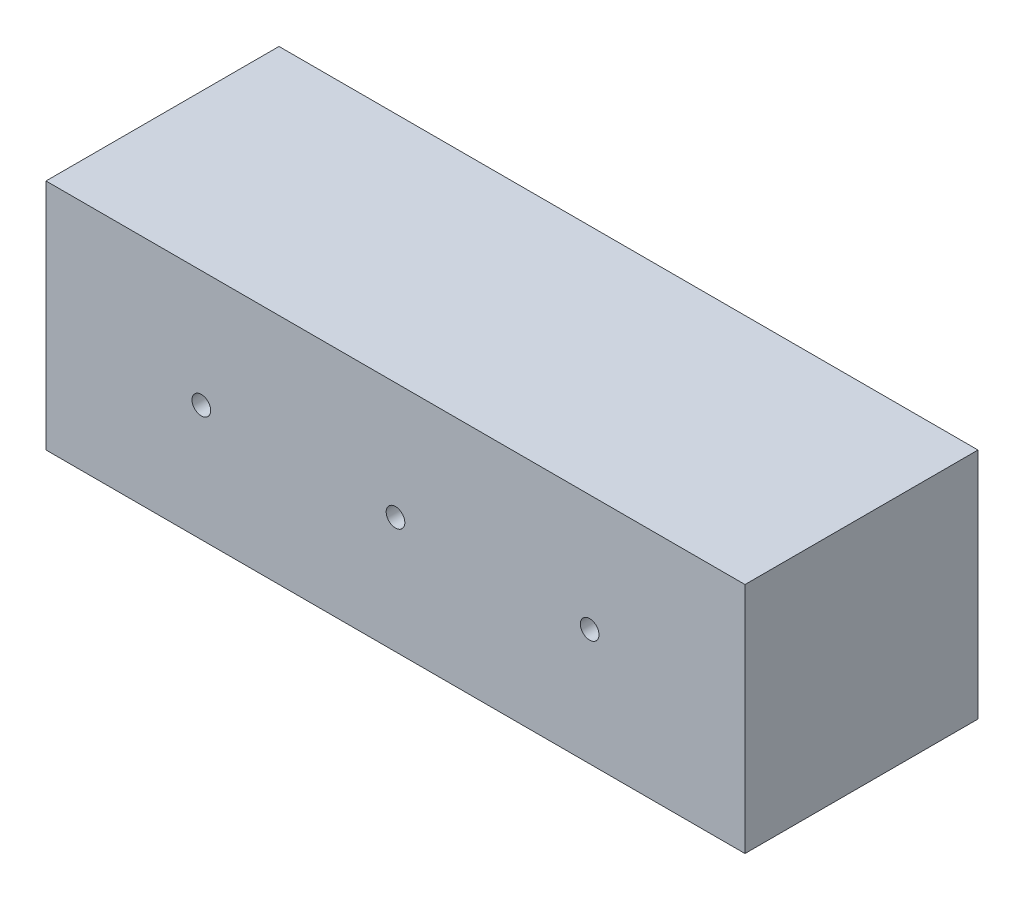
SolidWorks part; units mm, degrees
material "标准件"
ref_plane "前视基准面" through (0, 0, 0) normal (0, 0, 1) x (1, 0, 0)
ref_plane "上视基准面" through (0, 0, 0) normal (0, 1, 0) x (1, 0, 0)
ref_plane "右视基准面" through (0, 0, 0) normal (1, 0, 0) x (0, 0, -1)
sketch "草图1" plane through (0, 0, 0) normal (0, 1, 0) x (1, 0, 0)
  line L1 (-90, -30) -> (90, -30)
  line L2 (-90, -30) -> (-90, 30)
  line L3 (-90, 30) -> (90, 30)
  line L4 (90, -30) -> (90, 30)
  line L5 (-90, -30) -> (90, 30) construction
  line L6 (-90, 30) -> (90, -30) construction
  point P0 (0, 0)
  dimension "D1" = 180
  dimension "D2" = 60
extrude "凸台-拉伸1" add sketch "草图1" along normal blind 60
hole_wizard "M4 间隙孔1" positions "草图2" profile "草图3" hole size "M4" standard "ISO" end condition through all
sketch "草图2" plane through (0, 0, -30) normal (0, 0, -1) x (-1, 0, 0)
  line L0 (0, 60) -> (0, 0)
  line L1 (-90, 60) -> (90, 60) construction
  line L2 (-90, 0) -> (90, 0) construction
  line L3 (0, 30) -> (50, 30) construction
  point P0 (0, 30)
  point P13 (50, 30)
  point P16 (-50, 30)
  dimension "D1" = 2
  dimension "D2" = 50
sketch "草图3" plane through (0, 30, -30) normal (1, 0, 0) x (0, 1, 0)
  line L0 (0, 0) -> (0, 60)
  line L1 (0, 60) -> (2.4, 60)
  line L2 (2.4, 60) -> (2.4, 0)
  line L5 (2.4, 0) -> (0, 0)
  line L11 (0, -6.35) -> (0, 107.95) construction
  dimension "通孔孔直径" = 4.8
  dimension "通孔孔深度" = 60
